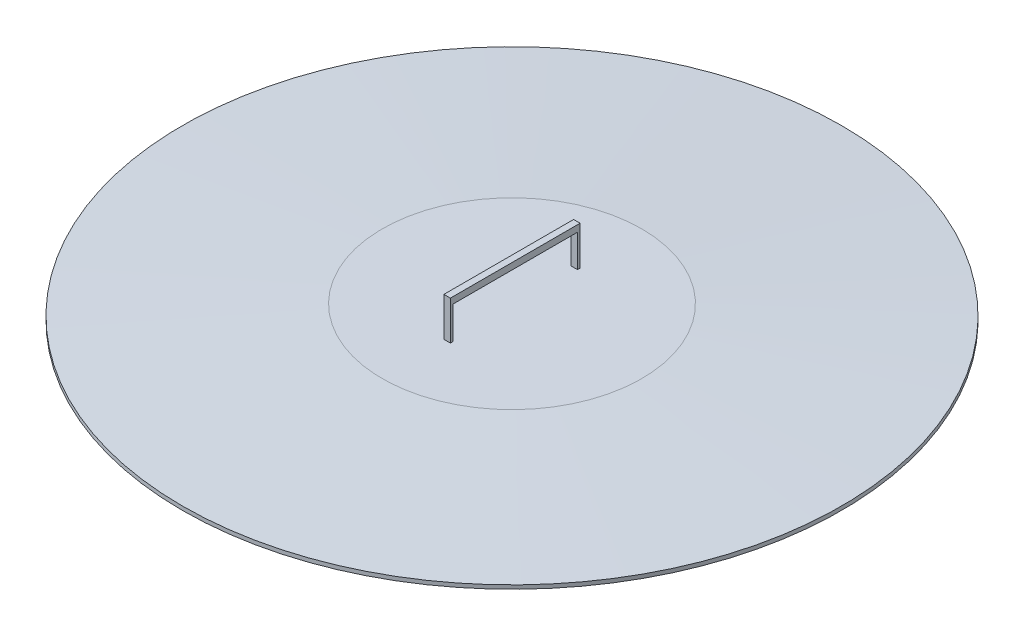
SolidWorks part; units mm, degrees
material "AISI 304"
ref_plane "Front Plane" through (0, 0, 0) normal (0, 0, 1) x (1, 0, 0)
ref_plane "Top Plane" through (0, 0, 0) normal (0, 1, 0) x (1, 0, 0)
ref_plane "Right Plane" through (0, 0, 0) normal (1, 0, 0) x (0, 0, -1)
sketch "Sketch1" plane through (0, 0, 0) normal (1, 0, 0) x (0, 0, -1)
  line L0 (0, 0) -> (0, 64.2209) construction
  line L1 (253, -0.6186) -> (253, 1.3814)
  line L2 (253, -0.6186) -> (254, -0.6186)
  line L3 (254, -0.6186) -> (254, 1.3814)
  line L4 (253, 1.3814) -> (99.9739, 9.3814)
  line L5 (254, 1.3814) -> (254, 2.3305)
  line L6 (254, 2.3305) -> (100, 10.3814)
  line L7 (0, 10.3814) -> (100, 10.3814)
  line L8 (0, 9.3814) -> (99.9739, 9.3814)
  line L9 (0, 10.3814) -> (0, 9.3814)
  dimension "D1" = 2
  dimension "D2" = 253
  dimension "D3" = 1
  dimension "D4" = 2
  dimension "D5" = 1
  dimension "D6" = 1
  dimension "D7" = 10
  dimension "D8" = 100
revolve "Revolve1" add sketch "Sketch1" angle 360 about L0
sketch "Sketch2" plane through (0, 0, 0) normal (1, 0, 0) x (0, 0, -1)
  line L0 (0, 0) -> (0, 35.3814) construction
  line L1 (-48, 10.3814) -> (-48, 35.3814)
  line L2 (100, 10.3814) -> (-100, 10.3814) construction
  line L3 (-48, 35.3814) -> (48, 35.3814)
  line L5 (50, 40.3814) -> (-50, 40.3814)
  line L6 (-50, 40.3814) -> (-50, 10.3814)
  line L7 (-50, 10.3814) -> (-48, 10.3814)
  line L8 (50, 40.3814) -> (50, 10.3814)
  line L9 (48, 10.3814) -> (48, 35.3814)
  line L10 (50, 10.3814) -> (48, 10.3814)
  line L11 (0, 40.3814) -> (0, 24.529) construction
  dimension "D1" = 50
  dimension "D2" = 2
  dimension "D3" = 30
  dimension "D4" = 25
extrude "Boss-Extrude2" add sketch "Sketch2" along normal mid plane 5
